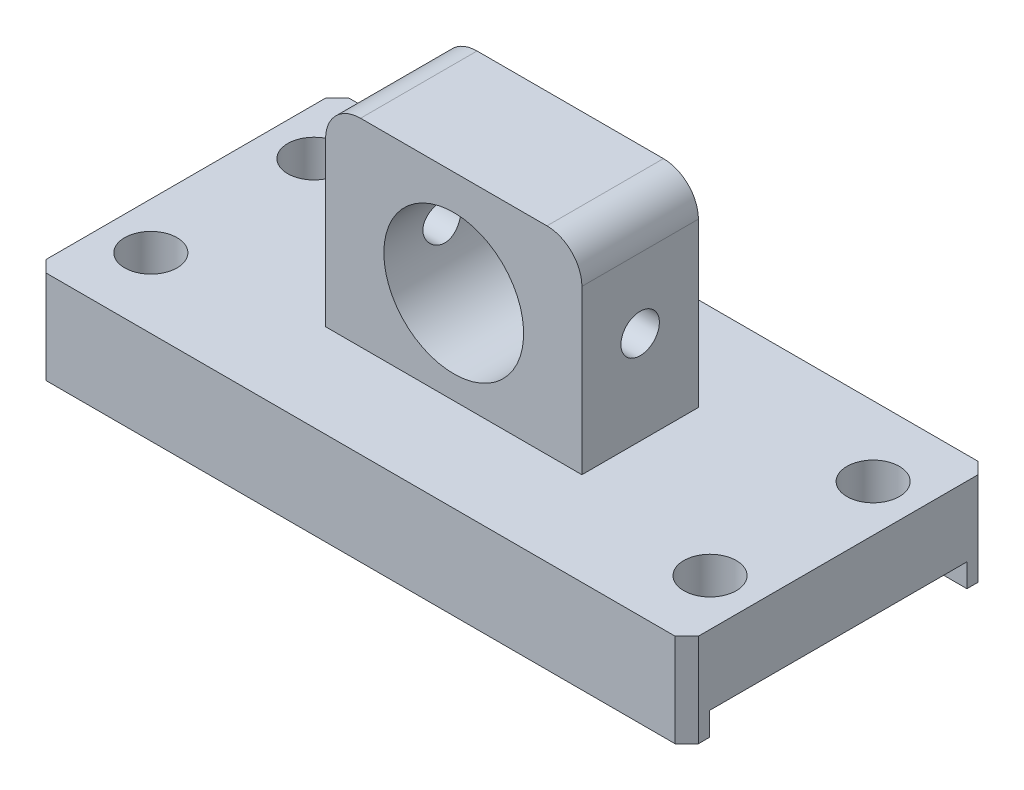
from build123d import *

# Parameters (mm, degrees)
SKETCH_1_W              = 56
SKETCH_1_H              = 26
EXTRUDE_1_DEPTH         = 8
SKETCH_2_W              = 70.031318806
SKETCH_2_H              = 22.1
CUT_EXTRUDE_1_DEPTH     = 2
SKETCH_3_W              = 22
SKETCH_3_H              = 10
EXTRUDE_2_DEPTH         = 17
SKETCH_4_R              = 6
CUT_EXTRUDE_2_DEPTH     = 46.661800227
HOLE_WIZARD_4_5_4_5_1_D = 4.5
FILLET_2_R              = 3
HOLE_WIZARD_M4_1_D      = 3.3
CHAMFER_1_SIZE          = 1


with BuildPart() as part:
    # 草图1 → 凸台-拉伸1 (new body)
    with BuildSketch(Plane(origin=(0, 0, 0), x_dir=(1, 0, 0), z_dir=(0, 1, 0))):
        Rectangle(SKETCH_1_W, SKETCH_1_H)
    extrude(amount=EXTRUDE_1_DEPTH)

    # 草图2 → 切除-拉伸1 (cut)
    with BuildSketch(Plane.XZ):
        Rectangle(SKETCH_2_W, SKETCH_2_H)
    extrude(amount=-CUT_EXTRUDE_1_DEPTH, mode=Mode.SUBTRACT)

    # 草图3 → 凸台-拉伸2 (add)
    with BuildSketch(Plane(origin=(0, 8, 0), x_dir=(1, 0, 0), z_dir=(0, 1, 0))):
        Rectangle(SKETCH_3_W, SKETCH_3_H)
    extrude(amount=EXTRUDE_2_DEPTH)

    # 草图4 → 切除-拉伸2 (cut, through all)
    with BuildSketch(Plane(origin=(0, 0, -13), x_dir=(-1, 0, 0), z_dir=(0, 0, -1))):
        with Locations((0, 16)):
            Circle(SKETCH_4_R)
    extrude(amount=-CUT_EXTRUDE_2_DEPTH, mode=Mode.SUBTRACT)

    # Ø4.5 (4.5) 直径孔1 (through all)
    with Locations(Plane(origin=(0, 8, 0), x_dir=(1, 0, 0), z_dir=(0, 1, 0))):
        with Locations((-24, 7), (-24, -7), (24, 7), (24, -7)):
            Hole(HOLE_WIZARD_4_5_4_5_1_D / 2)

    # 圆角2
    fillet_2_edges = [part.edges().sort_by_distance(p)[0] for p in [
        (11, 25, 0),
        (-11, 25, 0),
    ]]
    fillet(fillet_2_edges, radius=FILLET_2_R)

    # M4 螺纹孔1 (through all)
    with Locations(Plane(origin=(11, 0, 0), x_dir=(0, 0, -1), z_dir=(1, 0, 0))):
        with Locations((0, 16)):
            Hole(HOLE_WIZARD_M4_1_D / 2)

    # 倒角1
    chamfer_1_edges = [part.edges().sort_by_distance(p)[0] for p in [
        (28, 4, 13),
        (-28, 4, 13),
        (-28, 4, -13),
        (28, 4, -13),
    ]]
    chamfer(chamfer_1_edges, length=CHAMFER_1_SIZE)


solid = part.part
